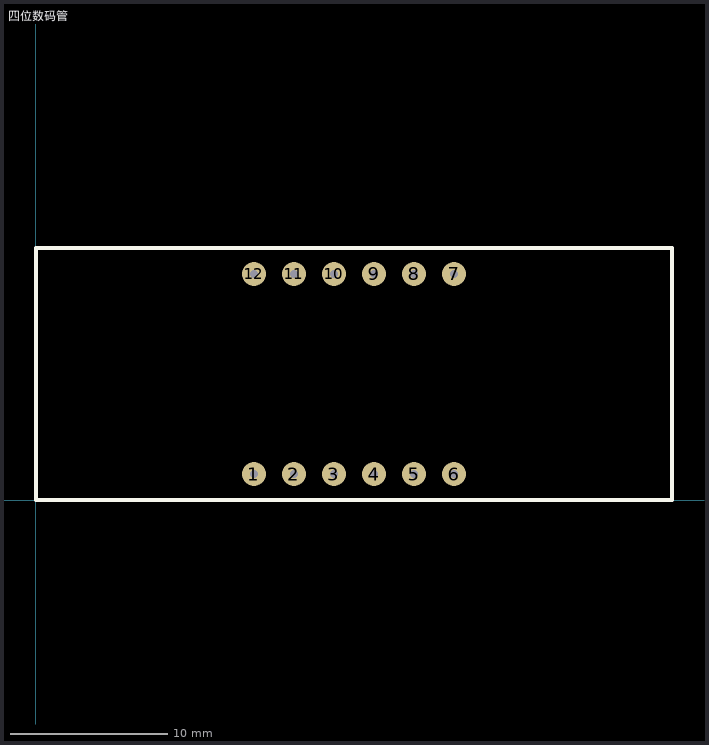
[diagram p0: the footprint, top view; thin cyan lines are the x and y axes]
# Altium footprint library MISC89340-20.PcbLib: 1 footprints
Each footprint in its own frame and in the unit in brackets; x right, y up, seen from the top. Pads: shape width x height; smd on the part's side, far side on the other; paste and mask are expansions set on the pad; w line width, h text height; cw(c..) or ccw(c..) is an arc to the next point about the centre after c.

## 四位数码管 [mm]
pads (12):
  round 1.524 hole 0.51: 1(13.85,1.65) 2(16.39,1.65) 3(18.93,1.65) 4(21.47,1.65) 5(24.01,1.65) 6(26.55,1.65) 7(26.55,14.35) 8(24.01,14.35) 9(21.47,14.35) 10(18.93,14.35) 11(16.39,14.35) 12(13.85,14.35)
Top Overlay:
  lines w0.254: 40.386,16 0,16 0,0 40.4,0 40.4,16